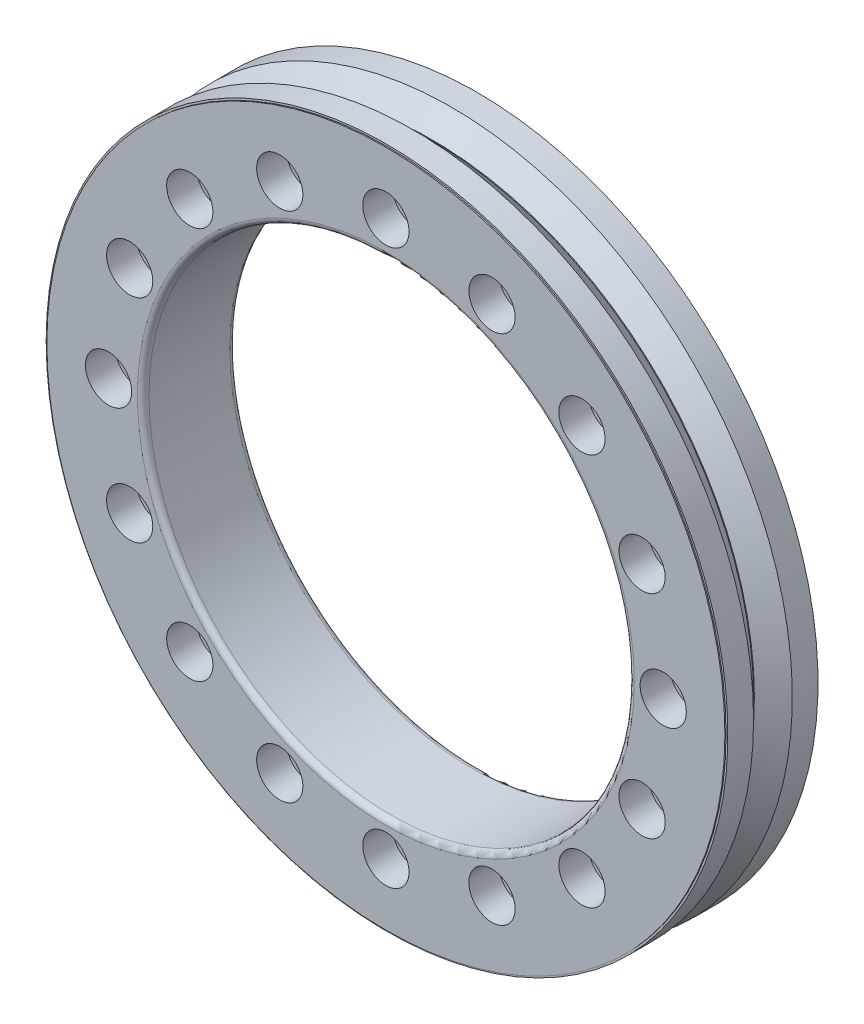
from build123d import *

# Parameters (mm, degrees)
SKETCH_1_R                = 147.5
SKETCH_1_R_2              = 105
EXTRUDE_1_DEPTH           = 20
HOLE_WIZARD_2_D           = 14
HOLE_WIZARD_2_CBORE_D     = 20
HOLE_WIZARD_2_CBORE_DEPTH = 13
PATTERN_CIRCULAR_1_COUNT  = 16
CUT_EXTRUDE_START         = -0.5
SKETCH_6_R                = 147.5
SKETCH_6_R_2              = 146.7
CUT_EXTRUDE_1_DEPTH       = 0.5
FILLET_1_R                = 2.5


with BuildPart() as part:
    # 草图1 → 凸台-拉伸1 (new, symmetric)
    with BuildSketch(Plane.XY):
        Circle(SKETCH_1_R)
        Circle(SKETCH_1_R_2, mode=Mode.SUBTRACT)
    extrude(amount=EXTRUDE_1_DEPTH, both=True)

    # 打孔尺寸(%根据)内六角圆柱头螺钉的类型2 (through all)
    with Locations(Plane.XY.offset(20)):
        with Locations((0, 120)):
            hole_wizard_2 = CounterBoreHole(HOLE_WIZARD_2_D / 2, HOLE_WIZARD_2_CBORE_D / 2, HOLE_WIZARD_2_CBORE_DEPTH)

    # 阵列(圆周)1: 打孔尺寸(%根据)内六角圆柱头螺钉的类型2 ×16 about axis
    pattern_circular_1_axis = Axis((0, 0, 0), (0, 0, 1))
    for i in range(1, PATTERN_CIRCULAR_1_COUNT):
        add(hole_wizard_2.rotate(pattern_circular_1_axis, i * 360 / PATTERN_CIRCULAR_1_COUNT), mode=Mode.SUBTRACT)

    # 草图5 → 切除-旋转1 (revolve, cut)
    with BuildSketch(Plane(origin=(0, 0, 0), x_dir=(1, 0, 0), z_dir=(0, 1, 0))):
        with BuildLine():
            Line((139.291495321, 0.176776695), (147.6, 8.485281374))
            Line((147.6, 8.485281374), (147.6, -8.485281374))
            Line((147.6, -8.485281374), (139.291495321, -0.176776695))
            ThreePointArc((139.291495321, -0.176776695), (138.864718626, 0), (139.291495321, 0.176776695))
        make_face()
    revolve(axis=Axis((0, 0, 20), (0, 0, -1)), mode=Mode.SUBTRACT)

    # 草图6 → 切除-拉伸1 (cut)
    with BuildSketch(Plane(origin=(0, 0, -20), x_dir=(-1, 0, 0), z_dir=(0, 0, -1)).offset(CUT_EXTRUDE_START)):
        Circle(SKETCH_6_R)
        Circle(SKETCH_6_R_2, mode=Mode.SUBTRACT)
    cut_extrude_1 = extrude(amount=CUT_EXTRUDE_1_DEPTH, mode=Mode.SUBTRACT)

    # 镜向1: 切除-拉伸1 across plane
    add(cut_extrude_1.mirror(Plane.XY), mode=Mode.SUBTRACT)

    # 圆角1
    fillet_1_edges = [part.edges().sort_by_distance(p)[0] for p in [
        (-105, 0, -20),
        (-105, 0, 20),
    ]]
    fillet(fillet_1_edges, radius=FILLET_1_R)


solid = part.part
